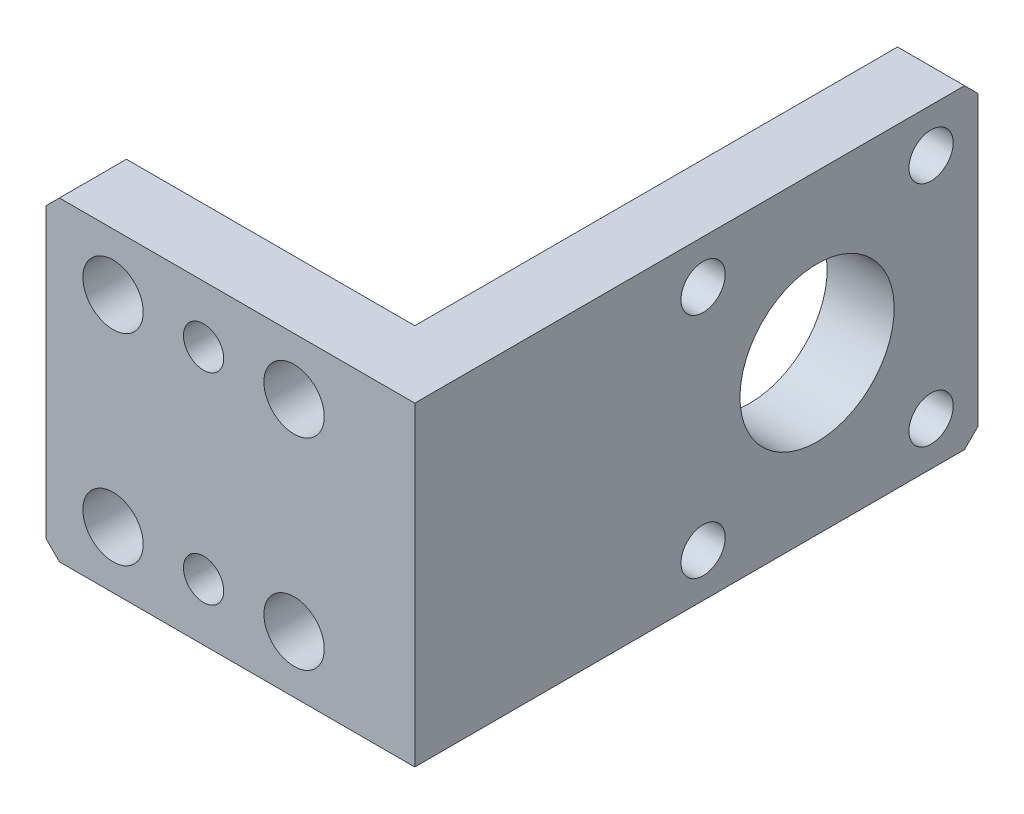
from build123d import *

# Parameters (mm, degrees)
SKETCH1_W                    = 55
SKETCH1_H                    = 47
BOSS_EXTRUDE1_DEPTH          = 10
SKETCH4_W                    = 10
SKETCH4_H                    = 47
BOSS_EXTRUDE2_DEPTH          = 74
M8_CLEARANCE_HOLE1_D         = 9
M8_CLEARANCE_HOLE1_DEPTH     = 121
M8_CLEARANCE_HOLE1_TIP       = 2.703872786
CHAMFER1_SIZE                = 2
SKETCH8_R                    = 11.5
CUT_EXTRUDE1_DEPTH           = 30
CHAMFER2_SIZE                = 2
SIZE_MM_BLIND_DOWEL_HOLE_1_D = 6
CIRPATTERN1_COUNT            = 4


with BuildPart() as part:
    # Sketch1 → Boss-Extrude1 (new body)
    with BuildSketch(Plane.XY):
        Rectangle(SKETCH1_W, SKETCH1_H)
    extrude(amount=BOSS_EXTRUDE1_DEPTH)

    # Sketch4 → Boss-Extrude2 (add)
    with BuildSketch(Plane(origin=(0, 0, 0), x_dir=(-1, 0, 0), z_dir=(0, 0, -1))):
        with Locations((-22.5, 0)):
            Rectangle(SKETCH4_W, SKETCH4_H)
    extrude(amount=BOSS_EXTRUDE2_DEPTH)

    # M8 Clearance Hole1
    with Locations(Plane(origin=(0, 0, 0), x_dir=(-1, 0, 0), z_dir=(0, 0, -1))):
        with Locations((17.5, -15), (17.5, 15), (-9.5, -15), (-9.5, 15)):
            Hole(M8_CLEARANCE_HOLE1_D / 2, depth=M8_CLEARANCE_HOLE1_DEPTH)
            with Locations((0, 0, -(M8_CLEARANCE_HOLE1_DEPTH + M8_CLEARANCE_HOLE1_TIP / 2))):  # 118° drill point
                Cone(0, M8_CLEARANCE_HOLE1_D / 2, M8_CLEARANCE_HOLE1_TIP, mode=Mode.SUBTRACT)

    # Chamfer1
    chamfer1_edges = [part.edges().sort_by_distance(p)[0] for p in [
        (-27.5, -23.5, 5),
        (-27.5, 23.5, 5),
    ]]
    chamfer(chamfer1_edges, length=CHAMFER1_SIZE)

    # Sketch8 → Cut-Extrude1 (cut)
    with BuildSketch(Plane.ZY.offset(-17.5)):
        with Locations(Location((-50, 0, 0), (0, 0, 270))):
            Circle(SKETCH8_R)
    extrude(amount=-CUT_EXTRUDE1_DEPTH, mode=Mode.SUBTRACT)

    # Chamfer2
    chamfer2_edges = [part.edges().sort_by_distance(p)[0] for p in [
        (22.5, 23.5, -74),
        (22.5, -23.5, -74),
    ]]
    chamfer(chamfer2_edges, length=CHAMFER2_SIZE)

    # Size mm blind dowel hole 1 (through all)
    with Locations(Plane(origin=(0, 0, 0), x_dir=(-1, 0, 0), z_dir=(0, 0, -1))):
        with Locations((4, -15), (4, 15)):
            Hole(SIZE_MM_BLIND_DOWEL_HOLE_1_D / 2)

    # Sketch14 → Hole size (per socket head cap screw type)1 (revolve, cut)
    with BuildSketch(Plane(origin=(17.5, -17, -67), x_dir=(0, 0, 1), z_dir=(0, 1, 0))):
        Polygon((0, 0), (0, 34.732840043), (3.3, 32.75), (3.3, 5), (5.5, 5), (5.5, 0), align=None)
    hole_size_per_socket_head_cap_screw_typ = revolve(axis=Axis((11.15, -17, -67), (1, 0, 0)), mode=Mode.SUBTRACT)

    # CirPattern1: Hole size (per socket head cap screw type)1 ×4 about axis
    cirpattern1_axis = Axis((0, 0, -50), (1, 0, 0))
    for i in range(1, CIRPATTERN1_COUNT):
        add(hole_size_per_socket_head_cap_screw_typ.rotate(cirpattern1_axis, i * 360 / CIRPATTERN1_COUNT), mode=Mode.SUBTRACT)


solid = part.part
